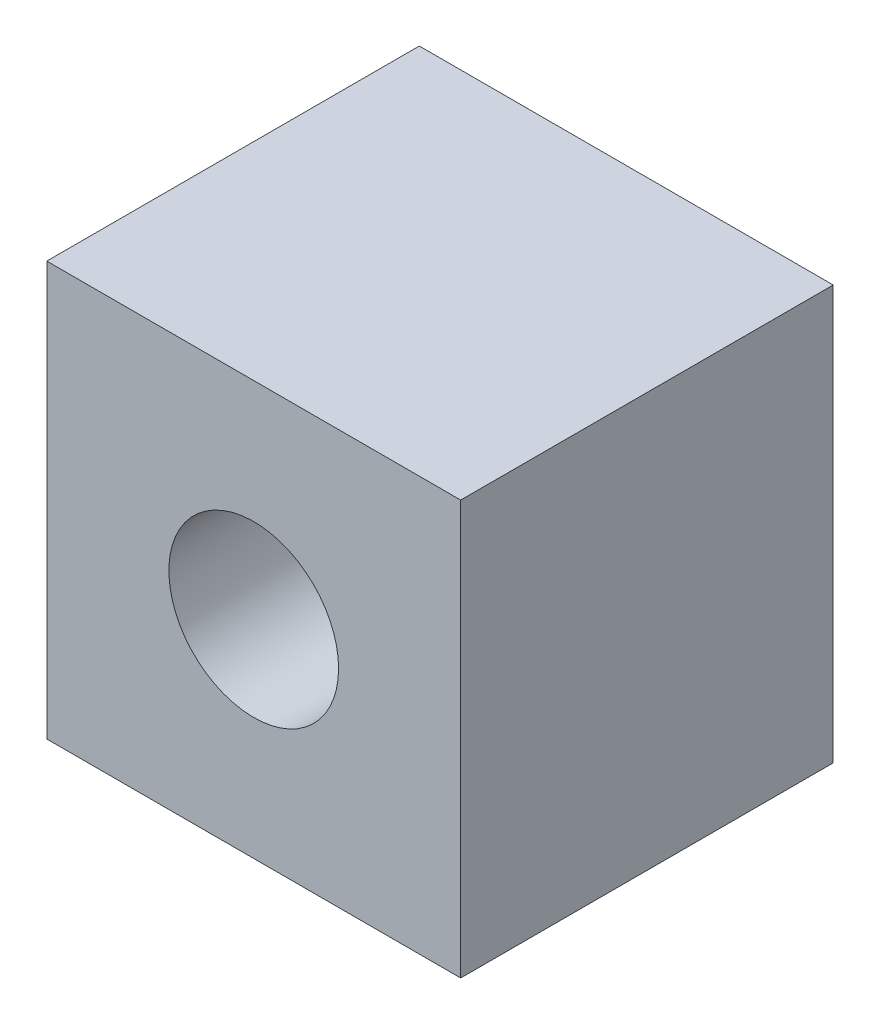
SolidWorks part; units mm, degrees
ref_plane "前视基准面" through (0, 0, 0) normal (0, 0, 1) x (1, 0, 0)
ref_plane "上视基准面" through (0, 0, 0) normal (0, 1, 0) x (1, 0, 0)
ref_plane "右视基准面" through (0, 0, 0) normal (1, 0, 0) x (0, 0, -1)
other "Configuration Table"
sketch "草图1" plane through (0, 0, 0) normal (0, 0, 1) x (1, 0, 0)
  line L0 (-20, -20) -> (20, -20)
  line L1 (20, -20) -> (20, 20)
  line L2 (20, 20) -> (-20, 20)
  line L3 (-20, 20) -> (-20, -20)
  point P0 (0, 0)
  dimension "D1" = 20
  dimension "D2" = 40
  dimension "D3" = 20
  dimension "D4" = 40
extrude "凸台-拉伸1" add sketch "草图1" against normal mid plane 36
sketch "草图2" plane through (0, 0, 0) normal (0, 0, 1) x (1, 0, 0)
  circle A0 centre (0, 0) radius 8.2
  point P0 (0, 0)
  dimension "D1" = 16.4
extrude "切除-拉伸1" cut sketch "草图2" against normal mid plane 60
